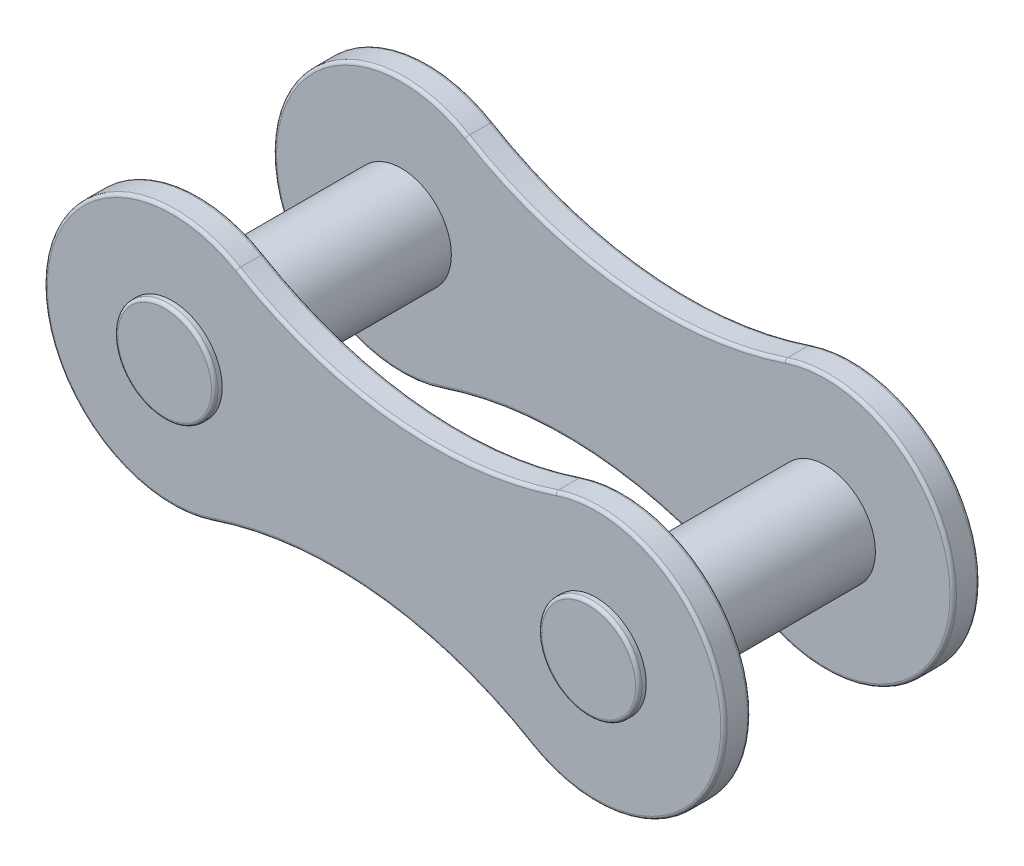
from build123d import *

# Parameters (mm, degrees)
BOSS_EXTRUDE1_START      = 4.75
SKETCH3_R                = 2.35
BOSS_EXTRUDE1_DEPTH      = 1.25
BOSS_EXTRUDE2_DEPTH      = 6.35
BOSS_EXTRUDE2_DEPTH_BACK = 6.35
SKETCH4_R                = 2.35
FILLET1_R                = 0.15
SCALE1_SCALE             = 0.5
SCALE2_SCALE             = 0.5
SCALE3_SCALE             = 0.5


with BuildPart() as part:
    # Sketch3 → Boss-Extrude1 (new body)
    with BuildSketch(Plane.XY.offset(BOSS_EXTRUDE1_START)):
        with BuildLine():
            ThreePointArc((-70.574575747, -5.382946104), (-61.545376441, -0.858174297), (-69.420828904, 5.464582104))
            ThreePointArc((-69.420828904, 5.464582104), (-77.051891637, 4.630059865), (-84.336698111, 7.0510391))
            ThreePointArc((-84.336698111, 7.0510391), (-93.365897416, 2.526267293), (-85.490444954, -3.796489108))
            ThreePointArc((-85.490444954, -3.796489108), (-77.85938222, -2.961966869), (-70.574575747, -5.382946104))
        make_face()
        with Locations((-87.399549733, 1.891684495)):
            Circle(SKETCH3_R, mode=Mode.SUBTRACT)
        with Locations((-67.511724124, -0.223591499)):
            Circle(SKETCH3_R, mode=Mode.SUBTRACT)
    extrude(amount=BOSS_EXTRUDE1_DEPTH)


with BuildPart() as body_2:
    # Mirror1: mirrored copy
    add(part.part.mirror(Plane.XY))


with BuildPart() as part_1:
    add(part.part)

    add(body_2.part)  # Boss-Extrude2 merges body 2
    # Sketch4 → Boss-Extrude2 (add, two sides: drawn at the far end of the back side and taken through both)
    with BuildSketch(Plane.XY.offset(-BOSS_EXTRUDE2_DEPTH_BACK)):
        with Locations((-67.511724124, -0.223591499)):
            Circle(SKETCH4_R)
        with Locations((-87.399549733, 1.891684495)):
            Circle(SKETCH4_R)
    extrude(amount=BOSS_EXTRUDE2_DEPTH + BOSS_EXTRUDE2_DEPTH_BACK)

    # Fillet1
    fillet1_edges = [part_1.edges().sort_by_distance(p)[0] for p in [
        (-77.051891637, 4.630059865, 6),
        (-93.365897416, 2.526267293, 6),
        (-69.861724124, -0.223591499, -6.35),
        (-69.861724124, -0.223591499, 6.35),
        (-77.85938222, -2.961966869, -4.75),
        (-61.545376441, -0.858174297, -4.75),
        (-77.051891637, 4.630059865, -4.75),
        (-93.365897416, 2.526267293, -4.75),
        (-77.85938222, -2.961966869, -6),
        (-61.545376441, -0.858174297, -6),
        (-77.051891637, 4.630059865, -6),
        (-93.365897416, 2.526267293, -6),
        (-89.749549733, 1.891684495, -6.35),
        (-89.749549733, 1.891684495, 6.35),
        (-77.85938222, -2.961966869, 6),
        (-93.365897416, 2.526267293, 4.75),
        (-77.051891637, 4.630059865, 4.75),
        (-61.545376441, -0.858174297, 4.75),
        (-77.85938222, -2.961966869, 4.75),
        (-61.545376441, -0.858174297, 6),
    ]]
    fillet(fillet1_edges, radius=FILLET1_R)


with BuildPart() as part_2:
    # Scale1: scaled about (-77.455636929, 0.834046498, 0)
    add(part_1.part.scale(SCALE1_SCALE).moved(Location((-38.727818464, 0.417023249, 0))))


with BuildPart() as part_3:
    # Scale2: scaled about (-77.455636929, 0.834046498, 0)
    add(part_2.part.scale(SCALE2_SCALE).moved(Location((-38.727818464, 0.417023249, 0))))


with BuildPart() as part_4:
    # Scale3: scaled about (-77.455636929, 0.834046498, 0)
    add(part_3.part.scale(SCALE3_SCALE).moved(Location((-38.727818464, 0.417023249, 0))))


solid = part_4.part
